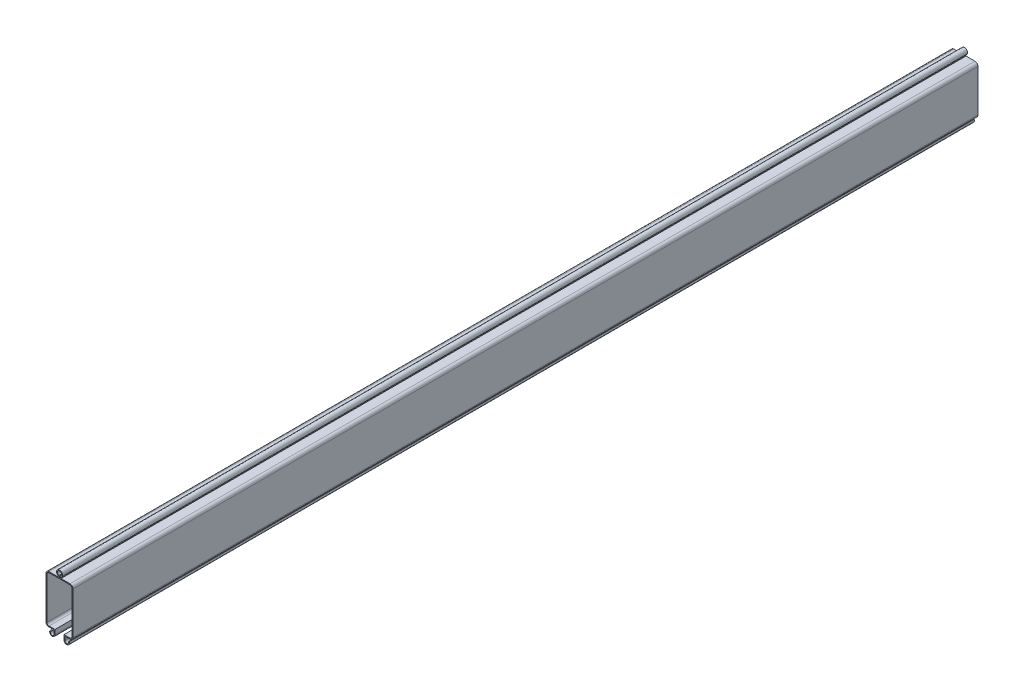
from build123d import *

# Parameters (mm, degrees)
BOSS_EXTRUDE1_DEPTH = 3017


with BuildPart() as part:
    # Sketch1 → Boss-Extrude1 (new body)
    with BuildSketch(Plane.XY):
        with BuildLine():
            Line((-35, 80), (-5, 80))
            Line((-5, 80), (-5, 83.719971064))
            ThreePointArc((-5, 83.719971064), (0, 102.380225102), (5, 83.719971064))
            Line((5, 83.719971064), (5, 80))
            Line((5, 80), (35, 80))
            ThreePointArc((35, 80), (42.071067812, 77.071067812), (45, 70))
            Line((45, 70), (45, -70))
            ThreePointArc((45, -70), (42.071067812, -77.071067812), (35, -80))
            Line((35, -80), (18, -80))
            Line((18, -80), (18, -92.395078412))
            ThreePointArc((18, -92.395078412), (25.155057115, -98.260822158), (29.503669933, -90.094344425))
            Line((29.503669933, -90.094344425), (32.272900703, -88.940498271))
            ThreePointArc((32.272900703, -88.940498271), (25.74340552, -101.202564185), (15, -92.395078412))
            Line((15, -92.395078412), (15, -77))
            Line((15, -77), (35, -77))
            ThreePointArc((35, -77), (39.949747468, -74.949747468), (42, -70))
            Line((42, -70), (42, 70))
            ThreePointArc((42, 70), (39.949747468, 74.949747468), (35, 77))
            Line((35, 77), (2, 77))
            Line((2, 77), (2, 85.672021169))
            ThreePointArc((2, 85.672021169), (0, 99.380225102), (-2, 85.672021169))
            Line((-2, 85.672021169), (-2, 77))
            Line((-2, 77), (-35, 77))
            ThreePointArc((-35, 77), (-39.949747468, 74.949747468), (-42, 70))
            Line((-42, 70), (-42, -70))
            ThreePointArc((-42, -70), (-39.949747468, -74.949747468), (-35, -77))
            Line((-35, -77), (-15, -77))
            Line((-15, -77), (-15, -92.395078412))
            ThreePointArc((-15, -92.395078412), (-25.74340552, -101.202564185), (-32.272900703, -88.940498271))
            Line((-32.272900703, -88.940498271), (-29.503669933, -90.094344425))
            ThreePointArc((-29.503669933, -90.094344425), (-25.155057115, -98.260822158), (-18, -92.395078412))
            Line((-18, -92.395078412), (-18, -80))
            Line((-18, -80), (-35, -80))
            ThreePointArc((-35, -80), (-42.071067812, -77.071067812), (-45, -70))
            Line((-45, -70), (-45, 70))
            ThreePointArc((-45, 70), (-42.071067812, 77.071067812), (-35, 80))
        make_face()
    extrude(amount=BOSS_EXTRUDE1_DEPTH)


solid = part.part
